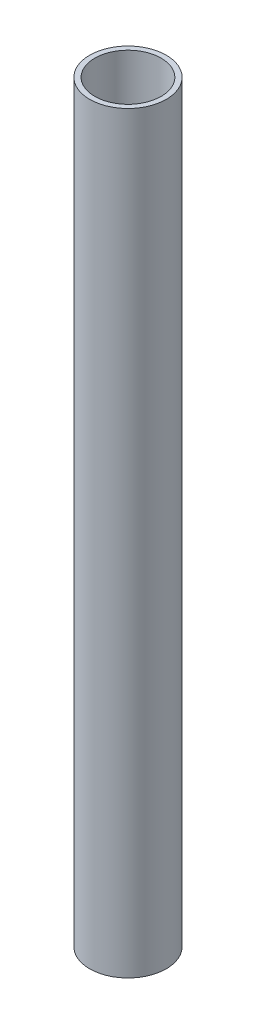
from build123d import *

# Parameters (mm, degrees)
SKETCH11_R                             = 30
SKETCH11_R_2                           = 26
GB_T_6728_2002_ROUND_TUBE_60_4_1_DEPTH = 590


with BuildPart() as part:
    # Sketch11 → Gb/t 6728-2002 round tube 60 × 4(1) (new body)
    with BuildSketch(Plane(origin=(0, 0, 0), x_dir=(-1, 0, 0), z_dir=(0, 1, 0))):
        Circle(SKETCH11_R)
        Circle(SKETCH11_R_2, mode=Mode.SUBTRACT)
    extrude(amount=GB_T_6728_2002_ROUND_TUBE_60_4_1_DEPTH)


solid = part.part
